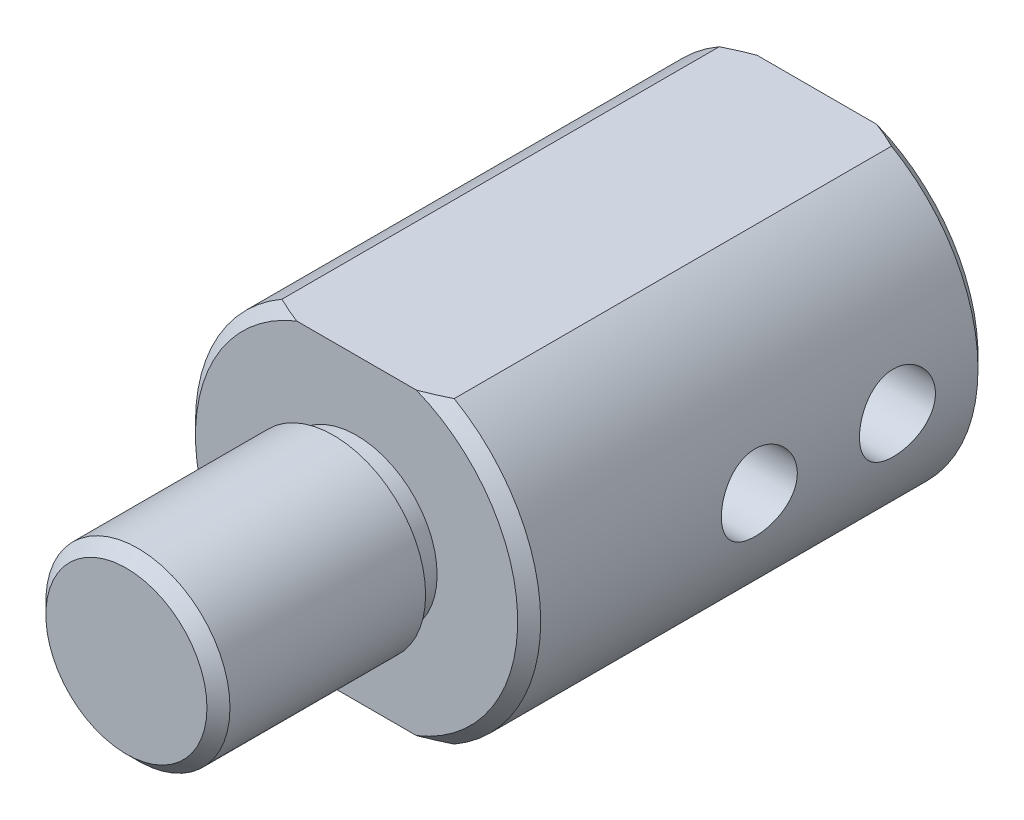
SolidWorks part; units mm, degrees
material "不锈钢304"
ref_plane "前视基准面" through (0, 0, 0) normal (0, 0, 1) x (1, 0, 0)
ref_plane "上视基准面" through (0, 0, 0) normal (0, 1, 0) x (1, 0, 0)
ref_plane "右视基准面" through (0, 0, 0) normal (1, 0, 0) x (0, 0, -1)
sketch "草图1" plane through (0, 0, 0) normal (0, 0, 1) x (1, 0, 0)
  circle A0 centre (0, 0) radius 7.5
  dimension "D1" = 15
extrude "凸台-拉伸1" add sketch "草图1" along normal blind 30
sketch "草图2" plane through (0, 0, 30) normal (0, 0, 1) x (1, 0, 0)
  circle A0 centre (0, 0) radius 4
  circle A1 centre (0, 0) radius 8.2263
  dimension "D1" = 8
extrude "切除-拉伸1" cut sketch "草图2" against normal blind 10
cosmetic thread "装饰螺纹线1" parameters "D1"=10, "D2"=7
sketch "草图3" plane through (0, 0, 0) normal (0, 0, -1) x (-1, 0, 0)
  circle A0 centre (0, 0) radius 1.5
  dimension "D1" = 3
extrude "切除-拉伸2" cut sketch "草图3" against normal blind 13
sketch "草图4" plane through (0, 0, 20) normal (0, 0, 1) x (1, 0, 0)
  circle A0 centre (0, 0) radius 4.4795
  circle A1 centre (0, 0) radius 3.5
  dimension "D1" = 7
extrude "切除-拉伸3" cut sketch "草图4" along normal blind 1
chamfer "倒角1" distance 0.5 angle 45 3 edges at (4, 0, 30) (7.5, 0, 20) (7.5, 0, 0)
hole_wizard "M4 螺纹孔1" positions "草图5" profile "草图6" tap size "M4" standard "GB"
sketch "草图5" plane through (0, 0, 0) normal (1, 0, 0) x (0, 0, -1)
  line L0 (0, -7) -> (0, 7) construction
  point P0 (-4, 0)
  point P2 (-10, 0)
  dimension "D1" = 6
  dimension "D2" = 4
cosmetic thread "孔螺蚊线2" parameters "D2"=4
sketch "草图6" plane through (0, 0, 4) normal (0, 1, 0) x (0, 0, 1)
  line L0 (0, 0) -> (0, 7.5)
  line L1 (0, 7.5) -> (1.65, 7.5)
  line L2 (1.65, 7.5) -> (1.65, 0)
  line L5 (1.65, 0) -> (0, 0)
  line L11 (0, -6.35) -> (0, 107.95) construction
  dimension "通孔螺纹孔钻头直径" = 3.3
  dimension "通孔螺纹孔钻头深度" = 7.5
cosmetic thread "孔螺蚊线3" parameters "D2"=4
sketch "草图7" plane through (0, 0, 0) normal (1, 0, 0) x (0, 0, -1)
  line L0 (0, 0) -> (7.0772, 0) construction
  line L1 (1.8131, 6.5) -> (-25.097, 6.5)
  line L2 (1.8131, 6.5) -> (1.8131, 11.3556)
  line L3 (1.8131, 11.3556) -> (-25.097, 11.3556)
  line L4 (-25.097, 6.5) -> (-25.097, 11.3556)
  line L5 (-21.7389, -6.5) -> (1.4047, -6.5)
  line L6 (-21.7389, -6.5) -> (-21.7389, -9.6312)
  line L7 (-21.7389, -9.6312) -> (1.4047, -9.6312)
  line L8 (1.4047, -6.5) -> (1.4047, -9.6312)
  dimension "D1" = 13
extrude "切除-拉伸4" cut sketch "草图7" against normal mid plane 10
